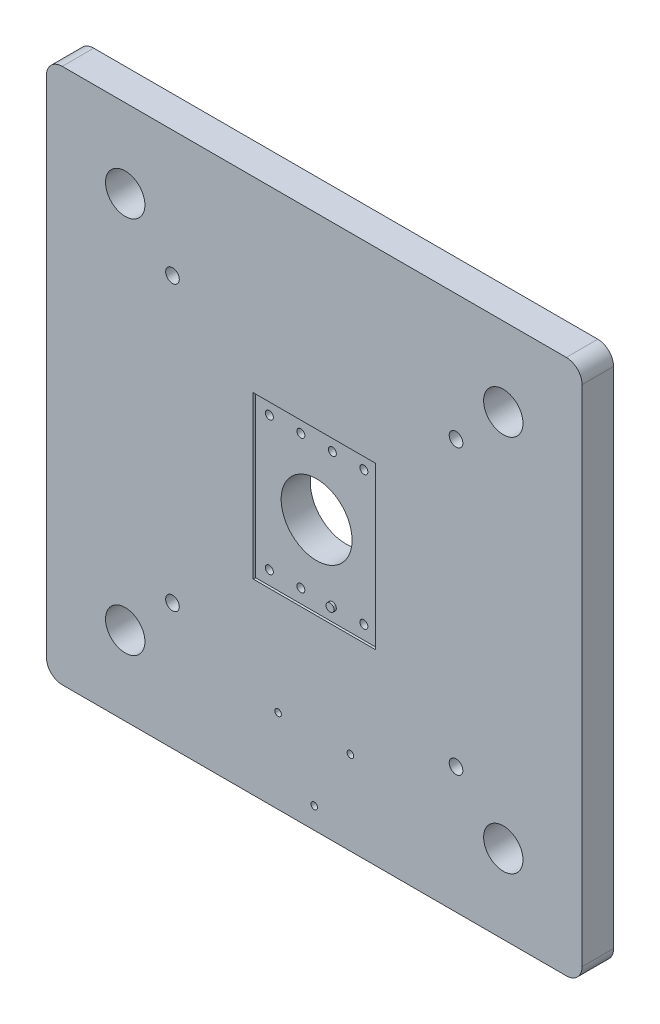
from build123d import *

# Parameters (mm, degrees)
SKETCH1_W           = 680
SKETCH1_H           = 680
BOSS_EXTRUDE1_DEPTH = 40
FILLET1_R           = 20
SKETCH2_W           = 155
SKETCH2_H           = 205
SKETCH2_R           = 5.05
CUT_EXTRUDE1_DEPTH  = 3
SKETCH3_R           = 5.05
CUT_EXTRUDE2_DEPTH  = 219
SKETCH4_R           = 45
CUT_EXTRUDE3_DEPTH  = 219
SKETCH5_R           = 8.65
CUT_EXTRUDE4_DEPTH  = 219
SKETCH6_R           = 4.2
CUT_EXTRUDE5_DEPTH  = 219
SKETCH7_R           = 25
CUT_EXTRUDE6_DEPTH  = 219


with BuildPart() as part:
    # Sketch1 → Boss-Extrude1 (new body)
    with BuildSketch(Plane.XY):
        Rectangle(SKETCH1_W, SKETCH1_H)
    extrude(amount=BOSS_EXTRUDE1_DEPTH)

    # Fillet1
    fillet1_edges = [part.edges().sort_by_distance(p)[0] for p in [
        (-340, 340, 20),
        (340, 340, 20),
        (340, -340, 20),
        (-340, -340, 20),
    ]]
    fillet(fillet1_edges, radius=FILLET1_R)

    # Sketch2 → Cut-Extrude1 (cut)
    with BuildSketch(Plane.XY.offset(40)):
        Rectangle(SKETCH2_W, SKETCH2_H)
        with Locations((-60, 85)):
            Circle(SKETCH2_R, mode=Mode.SUBTRACT)
        with Locations((-20, 85)):
            Circle(SKETCH2_R, mode=Mode.SUBTRACT)
        with Locations((20, 85)):
            Circle(SKETCH2_R, mode=Mode.SUBTRACT)
        with Locations((60, 85)):
            Circle(SKETCH2_R, mode=Mode.SUBTRACT)
        with Locations(Location((60, -85, 0), (0, 0, 180))):
            Circle(SKETCH2_R, mode=Mode.SUBTRACT)
        with Locations(Location((20, -85, 0), (0, 0, 180))):
            Circle(SKETCH2_R, mode=Mode.SUBTRACT)
        with Locations(Location((-20, -85, 0), (0, 0, 180))):
            Circle(SKETCH2_R, mode=Mode.SUBTRACT)
        with Locations(Location((-60, -85, 0), (0, 0, 180))):
            Circle(SKETCH2_R, mode=Mode.SUBTRACT)
    extrude(amount=-CUT_EXTRUDE1_DEPTH, mode=Mode.SUBTRACT)

    # Sketch3 → Cut-Extrude2 (cut)
    with BuildSketch(Plane.XY.offset(40)):
        with Locations(Location((-60, 85, 0), (0, 0, 180))):
            Circle(SKETCH3_R)
        with Locations(Location((-60, -85, 0), (0, 0, 180))):
            Circle(SKETCH3_R)
        with Locations(Location((-20, -85, 0), (0, 0, 180))):
            Circle(SKETCH3_R)
        with Locations(Location((60, -85, 0), (0, 0, 180))):
            Circle(SKETCH3_R)
        with Locations(Location((60, 85, 0), (0, 0, 180))):
            Circle(SKETCH3_R)
        with Locations(Location((20, 85, 0), (0, 0, 180))):
            Circle(SKETCH3_R)
        with Locations(Location((-20, 85, 0), (0, 0, 180))):
            Circle(SKETCH3_R)
    extrude(amount=-CUT_EXTRUDE2_DEPTH, mode=Mode.SUBTRACT)

    # Sketch4 → Cut-Extrude3 (cut)
    with BuildSketch(Plane.XY.offset(37)):
        Circle(SKETCH4_R)
    extrude(amount=-CUT_EXTRUDE3_DEPTH, mode=Mode.SUBTRACT)

    # Sketch5 → Cut-Extrude4 (cut)
    with BuildSketch(Plane.XY.offset(40)):
        with Locations((-180, 180)):
            Circle(SKETCH5_R)
        with Locations((180, 180)):
            Circle(SKETCH5_R)
        with Locations((180, -180)):
            Circle(SKETCH5_R)
        with Locations((-180, -180)):
            Circle(SKETCH5_R)
    extrude(amount=-CUT_EXTRUDE4_DEPTH, mode=Mode.SUBTRACT)

    # Sketch6 → Cut-Extrude5 (cut)
    with BuildSketch(Plane.XY.offset(40)):
        with Locations((0, -313)):
            Circle(SKETCH6_R)
        with Locations((45.899346401, -233.5)):
            Circle(SKETCH6_R)
        with Locations((-45.899346401, -233.5)):
            Circle(SKETCH6_R)
    extrude(amount=-CUT_EXTRUDE5_DEPTH, mode=Mode.SUBTRACT)

    # Sketch7 → Cut-Extrude6 (cut)
    with BuildSketch(Plane.XY.offset(40)):
        with Locations((-240, 240)):
            Circle(SKETCH7_R)
        with Locations((240, 240)):
            Circle(SKETCH7_R)
        with Locations((240, -240)):
            Circle(SKETCH7_R)
        with Locations((-240, -240)):
            Circle(SKETCH7_R)
    extrude(amount=-CUT_EXTRUDE6_DEPTH, mode=Mode.SUBTRACT)


solid = part.part
